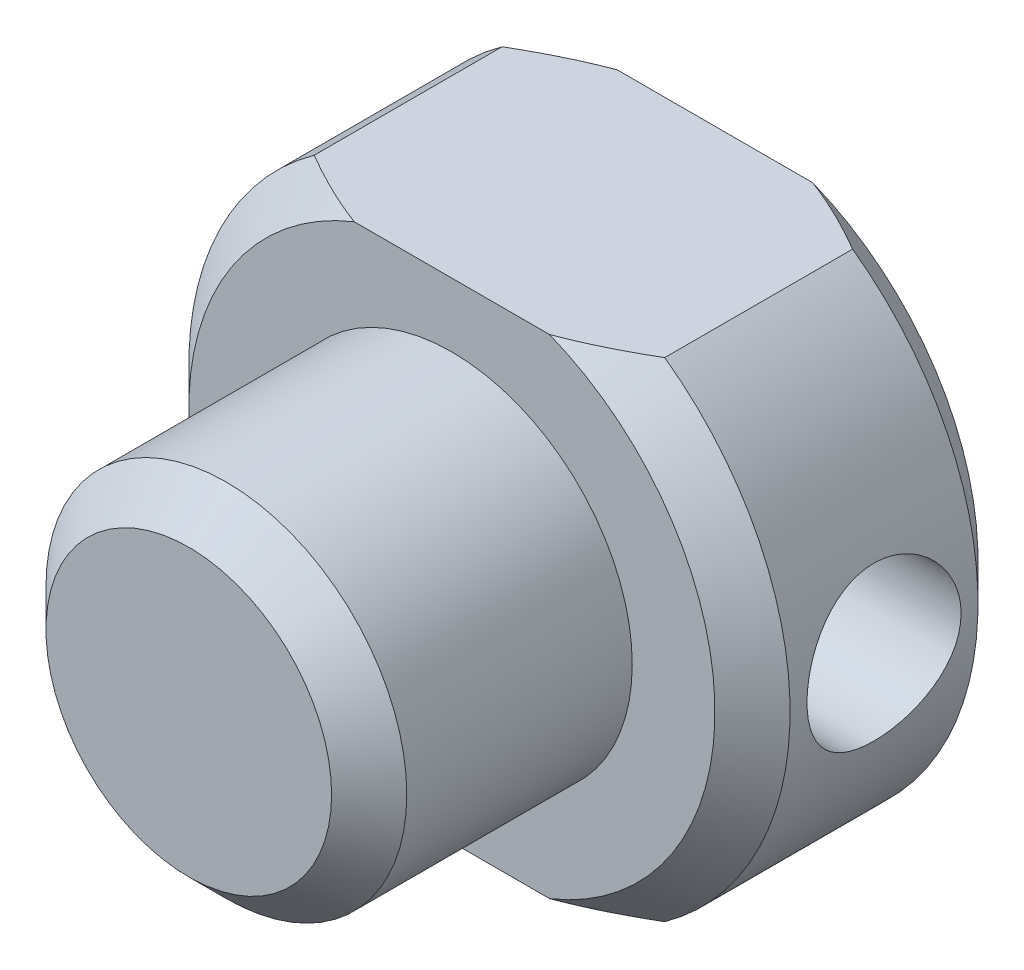
SolidWorks part; units mm, degrees
ref_plane "Front Plane" through (0, 0, 0) normal (0, 0, 1) x (1, 0, 0)
ref_plane "Top Plane" through (0, 0, 0) normal (0, 1, 0) x (1, 0, 0)
ref_plane "Right Plane" through (0, 0, 0) normal (1, 0, 0) x (0, 0, -1)
sketch "Sketch1" plane through (0, 0, 0) normal (0, 0, 1) x (1, 0, 0)
  circle A0 centre (0, 0) radius 4
  dimension "D1" = 8
extrude "Boss-Extrude1" add sketch "Sketch1" along normal blind 3.5
sketch "Sketch3" plane through (0, 0, 3.5) normal (0, 0, 1) x (1, 0, 0)
  circle A0 centre (0, 0) radius 2.4
  dimension "D1" = 4.8
extrude "Boss-Extrude2" add sketch "Sketch3" along normal blind 3.5
sketch "Sketch2" plane through (0, 0, 0) normal (0, 0, -1) x (-1, 0, 0)
  circle A0 centre (0, 0) radius 1.5
  dimension "D1" = 3
extrude "Cut-Extrude1" cut sketch "Sketch2" against normal blind 6
ref_plane "Plane1" through (4, 0, 0) normal (1, 0, 0) x (0, 0, -1)
hole_wizard "M2.5 Tapped Hole1" positions "Sketch5" profile "Sketch4" tap size "M2.5" standard "Gb"
sketch "Sketch5" plane through (4, 0, 0) normal (1, 0, 0) x (0, 0, -1)
  line L0 (0, 0) -> (-1.75, 0) construction
  point P0 (-1.75, 0)
  dimension "D1" = 1.75
cosmetic thread "Cosmetic thread 1" parameters "D2"=2.5
sketch "Sketch4" plane through (4, 0, 1.75) normal (0, 1, 0) x (0, 0, -1)
  line L0 (0, 0) -> (0, 2.5)
  line L1 (0, 2.5) -> (1.025, 2.5)
  line L2 (1.025, 2.5) -> (1.025, 0)
  line L5 (1.025, 0) -> (0, 0)
  line L11 (0, -6.35) -> (0, 107.95) construction
  dimension "通孔螺纹孔钻头直径" = 2.05
  dimension "通孔螺纹孔钻头深度" = 2.5
chamfer "Chamfer1" distance 0.5 angle 45 3 edges at (2.4, 0, 7) (4, 0, 3.5) (4, 0, 0)
sketch "Sketch6" plane through (0, 0, 3.5) normal (0, 0, 1) x (1, 0, 0)
  line L1 (-5.5971, 3.25) -> (5.5971, 3.25)
  line L2 (-5.5971, 3.25) -> (-5.5971, -3.25)
  line L3 (-5.5971, -3.25) -> (5.5971, -3.25)
  line L4 (5.5971, 3.25) -> (5.5971, -3.25)
  line L5 (-5.5971, 3.25) -> (5.5971, -3.25) construction
  line L6 (-5.5971, -3.25) -> (5.5971, 3.25) construction
  point P0 (0, 0)
  dimension "D1" = 6.5
extrude "Cut-Extrude2" cut sketch "Sketch6" against normal blind 10 flip side to cut
